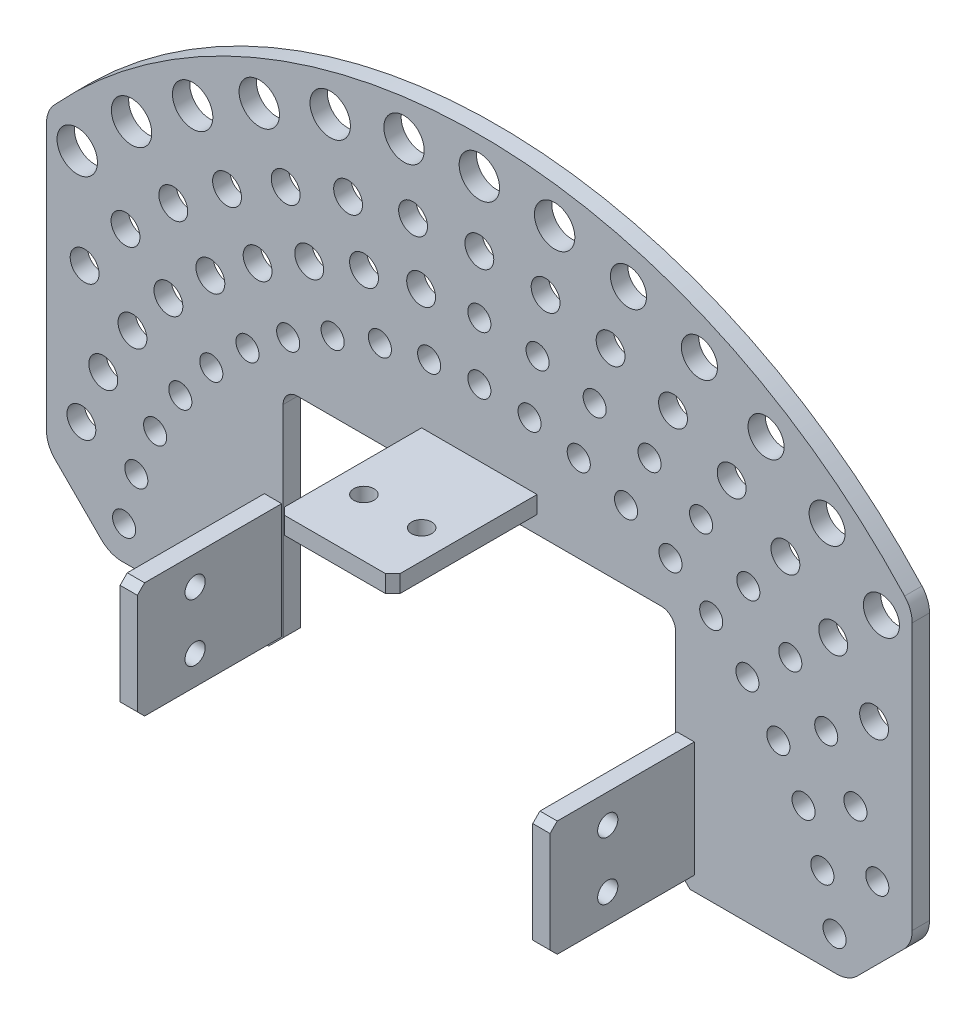
from build123d import *

# Parameters (mm, degrees)
EXTRUDE_1_DEPTH     = 12
FILLET_1_R          = 20
FILLET_2_R          = 10
SKETCH_2_W          = 12
SKETCH_2_H          = 80
EXTRUDE_2_DEPTH     = 100
EXTRUDE_2_2_DEPTH   = 100
SKETCH_2_W_2        = 80
SKETCH_2_H_2        = 12
EXTRUDE_2_3_DEPTH   = 100
SKETCH_3_R          = 7
CUT_EXTRUDE_1_DEPTH = 599.786272388
CHAMFER_1_SIZE      = 5
CHAMFER_2_SIZE      = 5
CHAMFER_3_SIZE      = 5
SKETCH_4_R          = 7
CUT_EXTRUDE_2_DEPTH = 491.974541091
SKETCH_5_R          = 14
SKETCH_5_R_2        = 12.5
CUT_EXTRUDE_3_DEPTH = 587.937816127
SKETCH_6_R          = 10
CUT_EXTRUDE_4_DEPTH = 50
SKETCH_7_R          = 8
SKETCH_7_R_2        = 10
CUT_EXTRUDE_5_DEPTH = 587.937816127
SKETCH_8_R          = 8
CUT_EXTRUDE_6_DEPTH = 50
CHAMFER_4_SIZE      = 10


with BuildPart() as part:
    # 草图1 → 凸台-拉伸1 (new body)
    with BuildSketch(Plane.XY):
        with BuildLine():
            Line((0, 0), (0, 160))
            Line((0, 160), (272, 160))
            Line((272, 160), (272, 0))
            Line((272, 0), (392, 0))
            Line((392, 0), (436, 44))
            Line((436, 44), (436, 244.575131106))
            ThreePointArc((436, 244.575131106), (136, 380), (-164, 244.575131106))
            Line((-164, 244.575131106), (-164, 44))
            Line((-164, 44), (-120, 0))
            Line((-120, 0), (0, 0))
        make_face()
    extrude(amount=EXTRUDE_1_DEPTH)

    # 圆角1
    fillet_1_edges = [part.edges().sort_by_distance(p)[0] for p in [
        (-120, 0, 6),
        (-164, 44, 6),
        (-164, 244.575131106, 6),
        (436, 244.575131106, 6),
        (436, 44, 6),
        (392, 0, 6),
    ]]
    fillet(fillet_1_edges, radius=FILLET_1_R)

    # 圆角2
    fillet_2_edges = [part.edges().sort_by_distance(p)[0] for p in [
        (272, 160, 6),
        (0, 160, 6),
    ]]
    fillet(fillet_2_edges, radius=FILLET_2_R)

    # 草图5 → 切除-拉伸3 (cut, through all)
    with BuildSketch(Plane.XY.offset(12)):
        with Locations((136, 355)):
            Circle(SKETCH_5_R)
        with Locations((188.18991286, 351.350525778)):
            Circle(SKETCH_5_R)
        with Locations(Location((-142.679309554, 230.923977385, 0), (0, 0, 180))):
            Circle(SKETCH_5_R)
        with Locations(Location((-105.045353632, 267.26666617, 0), (0, 0, 180))):
            Circle(SKETCH_5_R)
        with Locations(Location((-62.719724087, 298.018036059, 0), (0, 0, 180))):
            Circle(SKETCH_5_R)
        with Locations(Location((-16.526241153, 322.579546616, 0), (0, 0, 180))):
            Circle(SKETCH_5_R)
        with Locations(Location((32.635991569, 340.473135977, 0), (0, 0, 180))):
            Circle(SKETCH_5_R)
        with Locations(Location((83.81008714, 351.350525778, 0), (0, 0, 180))):
            Circle(SKETCH_5_R)
        with Locations((239.364008431, 340.473135977)):
            Circle(SKETCH_5_R_2)
        with Locations((288.526241153, 322.579546616)):
            Circle(SKETCH_5_R_2)
        with Locations((334.719724087, 298.018036059)):
            Circle(SKETCH_5_R_2)
        with Locations((377.045353632, 267.26666617)):
            Circle(SKETCH_5_R_2)
        with Locations((414.679309554, 230.923977385)):
            Circle(SKETCH_5_R_2)
    extrude(amount=-CUT_EXTRUDE_3_DEPTH, mode=Mode.SUBTRACT)

    # 草图6 → 切除-拉伸4 (cut)
    with BuildSketch(Plane.XY.offset(12)):
        with Locations((136, 310)):
            Circle(SKETCH_6_R)
        with Locations((181.927123317, 306.788462685)):
            Circle(SKETCH_6_R)
        with Locations((226.96032742, 297.21635966)):
            Circle(SKETCH_6_R)
        with Locations((270.223092215, 281.470001022)):
            Circle(SKETCH_6_R)
        with Locations((310.873357197, 259.855871732)):
            Circle(SKETCH_6_R)
        with Locations((348.119911197, 232.794666229)):
            Circle(SKETCH_6_R)
        with Locations((381.237792408, 200.813100098)):
            Circle(SKETCH_6_R)
        with Locations((-109.237792408, 200.813100098)):
            Circle(SKETCH_6_R)
        with Locations((-76.119911197, 232.794666229)):
            Circle(SKETCH_6_R)
        with Locations((-38.873357197, 259.855871732)):
            Circle(SKETCH_6_R)
        with Locations((1.776907785, 281.470001022)):
            Circle(SKETCH_6_R)
        with Locations((45.03967258, 297.21635966)):
            Circle(SKETCH_6_R)
        with Locations((90.072876683, 306.788462685)):
            Circle(SKETCH_6_R)
        with Locations((409.582398943, 164.533658145)):
            Circle(SKETCH_6_R)
        with Locations((-137.582398943, 164.533658145)):
            Circle(SKETCH_6_R)
    extrude(amount=-CUT_EXTRUDE_4_DEPTH, mode=Mode.SUBTRACT)

    # 草图7 → 切除-拉伸5 (cut, through all)
    with BuildSketch(Plane.XY.offset(12)):
        with Locations((136, 270)):
            Circle(SKETCH_7_R)
        with Locations((176.360199278, 267.177739935)):
            Circle(SKETCH_7_R)
        with Locations((215.934833187, 258.765891822)):
            Circle(SKETCH_7_R)
        with Locations((253.953626492, 244.928182716)):
            Circle(SKETCH_7_R)
        with Locations((289.676586628, 225.933947885)):
            Circle(SKETCH_7_R)
        with Locations((322.408406809, 202.152888505)):
            Circle(SKETCH_7_R)
        with Locations((351.511999388, 174.047875844)):
            Circle(SKETCH_7_R)
        with Locations((376.420896041, 142.165942007)):
            Circle(SKETCH_7_R)
        with Locations((396.650273427, 107.127632569)):
            Circle(SKETCH_7_R)
        with Locations((411.806389726, 69.614928369)):
            Circle(SKETCH_7_R)
        with Locations((95.639800722, 267.177739935)):
            Circle(SKETCH_7_R_2)
        with Locations((56.065166813, 258.765891822)):
            Circle(SKETCH_7_R_2)
        with Locations((18.046373508, 244.928182716)):
            Circle(SKETCH_7_R_2)
        with Locations((-17.676586628, 225.933947885)):
            Circle(SKETCH_7_R_2)
        with Locations((-50.408406809, 202.152888505)):
            Circle(SKETCH_7_R_2)
        with Locations((-79.511999388, 174.047875844)):
            Circle(SKETCH_7_R_2)
        with Locations((-104.420896041, 142.165942007)):
            Circle(SKETCH_7_R_2)
        with Locations((-124.650273427, 107.127632569)):
            Circle(SKETCH_7_R_2)
        with Locations((-139.806389726, 69.614928369)):
            Circle(SKETCH_7_R_2)
    extrude(amount=-CUT_EXTRUDE_5_DEPTH, mode=Mode.SUBTRACT)

    # 草图8 → 切除-拉伸6 (cut)
    with BuildSketch(Plane.XY.offset(12)):
        with Locations((136, 230)):
            Circle(SKETCH_8_R)
        with Locations((170.79327524, 227.567017185)):
            Circle(SKETCH_8_R)
        with Locations((204.909338954, 220.315423985)):
            Circle(SKETCH_8_R)
        with Locations((237.684160769, 208.386364411)):
            Circle(SKETCH_8_R)
        with Locations((268.479816058, 192.012024039)):
            Circle(SKETCH_8_R)
        with Locations((296.696902422, 171.51111078)):
            Circle(SKETCH_8_R)
        with Locations((321.786206369, 147.28265159)):
            Circle(SKETCH_8_R)
        with Locations((343.259393139, 119.798225868)):
            Circle(SKETCH_8_R)
        with Locations((360.698511575, 89.592786697)):
            Circle(SKETCH_8_R)
        with Locations((373.764129074, 57.254248594)):
            Circle(SKETCH_8_R)
        with Locations((382.201938253, 23.412044417)):
            Circle(SKETCH_8_R)
        with Locations((-110.201938253, 23.412044417)):
            Circle(SKETCH_8_R)
        with Locations((-101.764129074, 57.254248594)):
            Circle(SKETCH_8_R)
        with Locations((-88.698511575, 89.592786697)):
            Circle(SKETCH_8_R)
        with Locations((-71.259393139, 119.798225868)):
            Circle(SKETCH_8_R)
        with Locations((-49.786206369, 147.28265159)):
            Circle(SKETCH_8_R)
        with Locations((-24.696902422, 171.51111078)):
            Circle(SKETCH_8_R)
        with Locations((3.520183942, 192.012024039)):
            Circle(SKETCH_8_R)
        with Locations((34.315839231, 208.386364411)):
            Circle(SKETCH_8_R)
        with Locations((67.090661046, 220.315423985)):
            Circle(SKETCH_8_R)
        with Locations((101.20672476, 227.567017185)):
            Circle(SKETCH_8_R)
    extrude(amount=-CUT_EXTRUDE_6_DEPTH, mode=Mode.SUBTRACT)

    # 倒角4
    chamfer_4_edges = [part.edges().sort_by_distance(p)[0] for p in [
        (272, 0, 6),
        (0, 0, 6),
    ]]
    chamfer(chamfer_4_edges, length=CHAMFER_4_SIZE)


with BuildPart() as body_2:
    # 草图2 → 凸台-拉伸2 (new body)
    with BuildSketch(Plane.XY.offset(12)):
        with Locations((-7, 50)):
            Rectangle(SKETCH_2_W, SKETCH_2_H)
    extrude(amount=EXTRUDE_2_DEPTH)


with BuildPart() as body_3:
    # 草图2 → Extrude 2 2 (new body)
    with BuildSketch(Plane.XY.offset(12)):
        with Locations((279, 50)):
            Rectangle(SKETCH_2_W, SKETCH_2_H)
    extrude(amount=EXTRUDE_2_2_DEPTH)


with BuildPart() as body_4:
    # 草图2 → Extrude 2 3 (new body)
    with BuildSketch(Plane.XY.offset(12)):
        with Locations((136, 178)):
            Rectangle(SKETCH_2_W_2, SKETCH_2_H_2)
    extrude(amount=EXTRUDE_2_3_DEPTH)

    # 倒角3
    chamfer_3_edges = [body_4.edges().sort_by_distance(p)[0] for p in [
        (96, 178, 112),
        (176, 178, 112),
    ]]
    chamfer(chamfer_3_edges, length=CHAMFER_3_SIZE)

    # 草图4 → 切除-拉伸2 (cut, through all)
    with BuildSketch(Plane(origin=(0, 184, 0), x_dir=(1, 0, 0), z_dir=(0, 1, 0))):
        with Locations(Location((116, -72, 0), (0, 0, 270))):
            Circle(SKETCH_4_R)
        with Locations(Location((156, -72, 0), (0, 0, 270))):
            Circle(SKETCH_4_R)
    extrude(amount=-CUT_EXTRUDE_2_DEPTH, mode=Mode.SUBTRACT)


with BuildPart() as cut_extrude_1_tool:
    # 草图3 → 切除-拉伸1 (new, through all)
    with BuildSketch(Plane.ZY.offset(13)):
        with Locations(Location((72, 70, 0), (0, 0, 270))):
            Circle(SKETCH_3_R)
        with Locations(Location((72, 30, 0), (0, 0, 270))):
            Circle(SKETCH_3_R)
    extrude(amount=-CUT_EXTRUDE_1_DEPTH)


with BuildPart() as body_2_1:
    add(body_2.part)

    # 切除-拉伸1: cut by cut_extrude_1_tool
    add(cut_extrude_1_tool.part, mode=Mode.SUBTRACT)

    # 倒角1
    chamfer_1_edges = [body_2_1.edges().sort_by_distance(p)[0] for p in [
        (-7, 10, 112),
        (-7, 90, 112),
    ]]
    chamfer(chamfer_1_edges, length=CHAMFER_1_SIZE)


with BuildPart() as body_3_1:
    add(body_3.part)

    # 切除-拉伸1: cut by cut_extrude_1_tool
    add(cut_extrude_1_tool.part, mode=Mode.SUBTRACT)

    # 倒角2
    chamfer_2_edges = [body_3_1.edges().sort_by_distance(p)[0] for p in [
        (279, 10, 112),
        (279, 90, 112),
    ]]
    chamfer(chamfer_2_edges, length=CHAMFER_2_SIZE)


solid = Compound([part.part, body_4.part, body_2_1.part, body_3_1.part])
